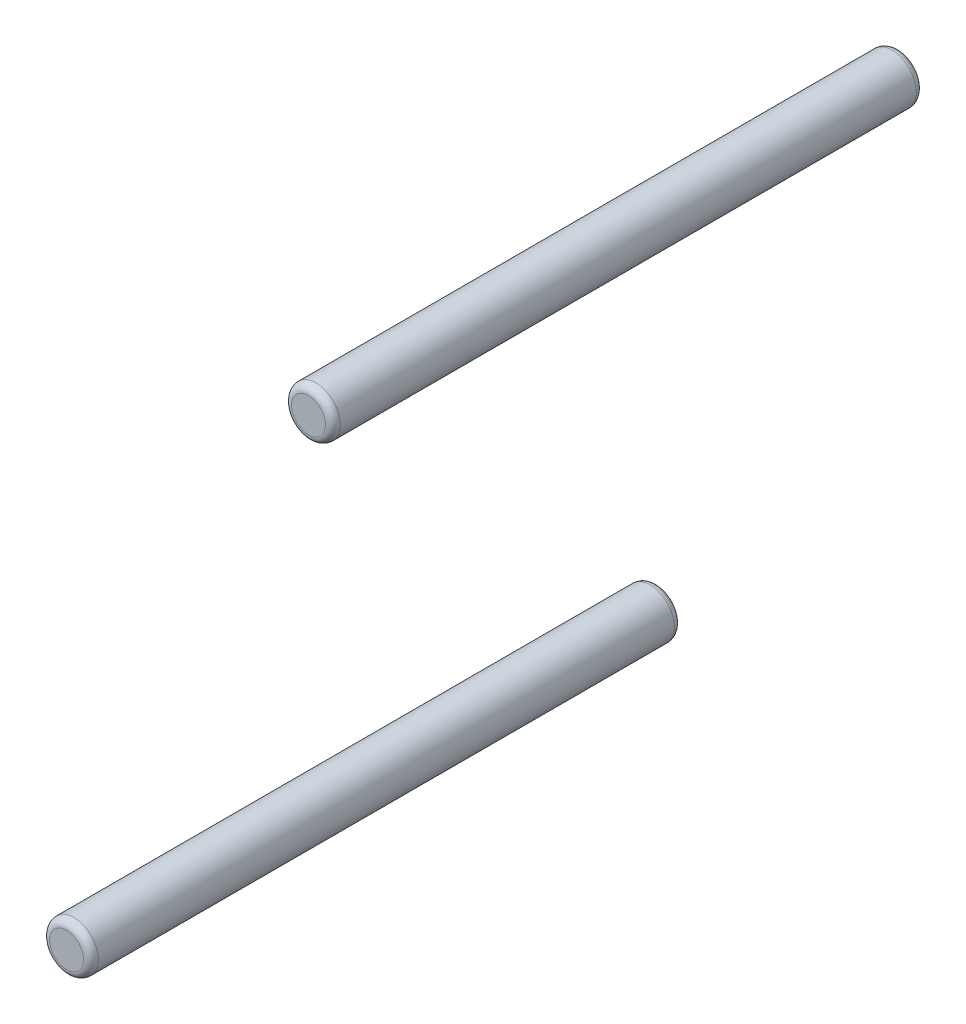
from build123d import *

# Parameters (mm, degrees)
SKETCH1_R             = 3.3
BOSS_EXTRUDE1_DEPTH   = 80
BOSS_EXTRUDE1_2_DEPTH = 80
FILLET1_R             = 1
FILLET2_R             = 1


with BuildPart() as part:
    # Sketch1 → Boss-Extrude1 (new body)
    with BuildSketch(Plane.XY):
        with Locations((-16.378850905, -39.542043991)):
            Circle(SKETCH1_R)
    extrude(amount=BOSS_EXTRUDE1_DEPTH)

    # Fillet1
    fillet1_edges = [part.edges().sort_by_distance(p)[0] for p in [
        (-19.678850905, -39.542043991, 0),
        (-19.678850905, -39.542043991, 80),
    ]]
    fillet(fillet1_edges, radius=FILLET1_R)


with BuildPart() as body_2:
    # Sketch1 → Boss-Extrude1 2 (new body)
    with BuildSketch(Plane.XY):
        with Locations((16.378850905, 39.542043991)):
            Circle(SKETCH1_R)
    extrude(amount=BOSS_EXTRUDE1_2_DEPTH)

    # Fillet2
    fillet2_edges = [body_2.edges().sort_by_distance(p)[0] for p in [
        (13.078850905, 39.542043991, 0),
        (13.078850905, 39.542043991, 80),
    ]]
    fillet(fillet2_edges, radius=FILLET2_R)


solid = Compound([part.part, body_2.part])
